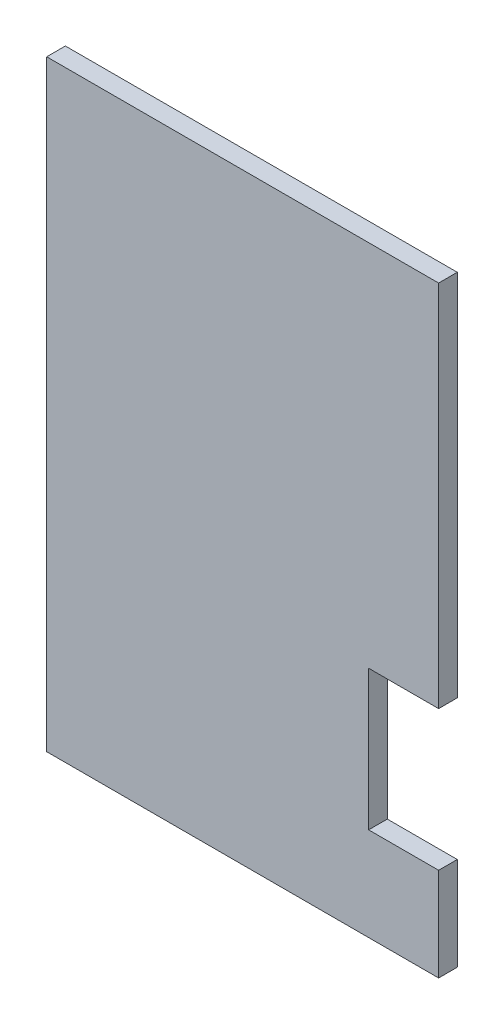
SolidWorks part; units mm, degrees
material "Q235B"
ref_plane "Front Plane" through (0, 0, 0) normal (0, 0, 1) x (1, 0, 0)
ref_plane "Top Plane" through (0, 0, 0) normal (0, 1, 0) x (1, 0, 0)
ref_plane "Right Plane" through (0, 0, 0) normal (1, 0, 0) x (0, 0, -1)
sketch "Sketch1" plane through (0, 0, 0) normal (0, 0, 1) x (1, 0, 0)
  line L0 (0, 0) -> (840, 0)
  line L1 (840, 500) -> (840, 1290)
  line L2 (840, 1290) -> (0, 1290)
  line L4 (0, 1290) -> (0, 0)
  line L5 (690, 200) -> (690, 500)
  line L6 (690, 500) -> (840, 500)
  line L7 (690, 200) -> (840, 200)
  line L8 (840, 200) -> (840, 0)
  dimension "D1" = 200
  dimension "D3" = 1290
  dimension "D5" = 500
  dimension "D6" = 150
  dimension "D8" = 840
extrude "Boss-Extrude1" add sketch "Sketch1" along normal blind 40
